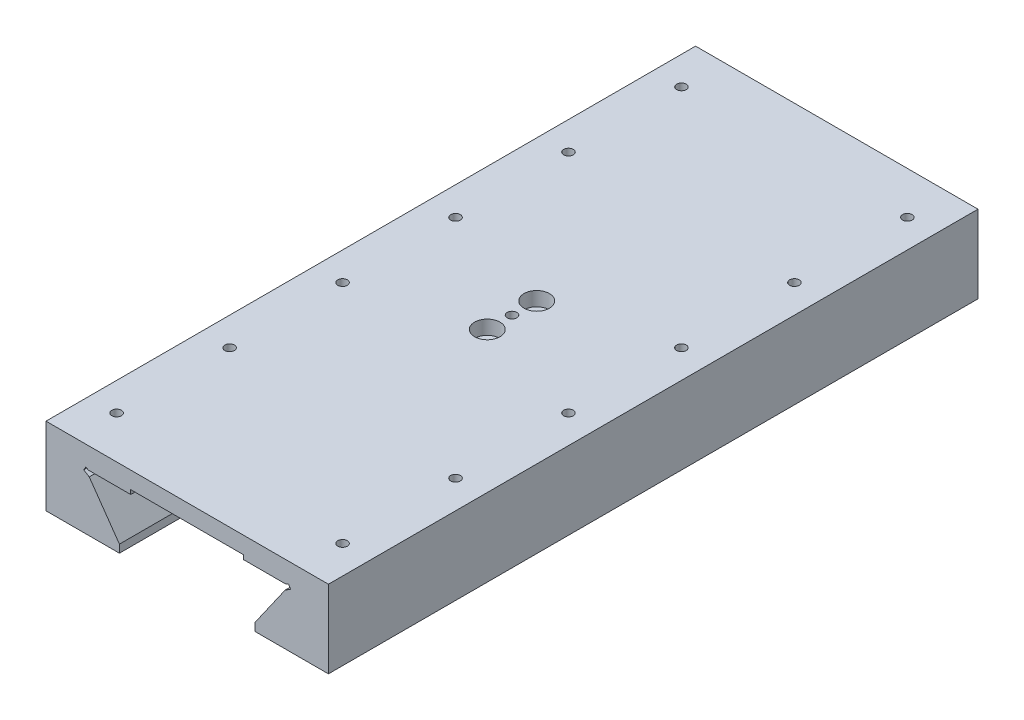
from build123d import *

# Parameters (mm, degrees)
BOSS_EXTRUDE1_DEPTH                     = 460
CBORE_FOR_M8_HEX_HEAD_BOLT1_D           = 9
CBORE_FOR_M8_HEX_HEAD_BOLT1_CBORE_D     = 18
CBORE_FOR_M8_HEX_HEAD_BOLT1_CBORE_DEPTH = 10
M8_TAPPED_HOLE1_D                       = 6.8
M8_TAPPED_HOLE1_DEPTH                   = 19.75
M8_TAPPED_HOLE1_TIP                     = 2.042926105


with BuildPart() as part:
    # Sketch1 → Boss-Extrude1 (new body)
    with BuildSketch(Plane.XY):
        Polygon((-40, 52.5), (-40, 55.5), (40, 55.5), (40, 52.5), (70, 52.5), (71.711448084, 53.534864946), (73.263745503, 50.96769282), (69.385770597, 48.622789502), (48, 18.080743852), (48, 12.5), (100, 12.5), (100, 67.5), (-100, 67.5), (-100, 12.5), (-48, 12.5), (-48, 18.080743852), (-69.385770597, 48.622789502), (-73.263745503, 50.96769282), (-71.711448084, 53.534864946), (-70, 52.5), align=None)
    extrude(amount=-BOSS_EXTRUDE1_DEPTH)

    # CBORE for M8 Hex Head Bolt1 (through all)
    with Locations(Plane(origin=(0, 67.5, 0), x_dir=(1, 0, 0), z_dir=(0, 1, 0))):
        with Locations((0, 247.5), (0, 212.5)):
            CounterBoreHole(CBORE_FOR_M8_HEX_HEAD_BOLT1_D / 2, CBORE_FOR_M8_HEX_HEAD_BOLT1_CBORE_D / 2, CBORE_FOR_M8_HEX_HEAD_BOLT1_CBORE_DEPTH)

    # M8 Tapped Hole1
    with Locations(Plane(origin=(0, 67.5, 0), x_dir=(1, 0, 0), z_dir=(0, 1, 0))):
        with Locations((1.4e-07, 230), (80.000000279, 430), (-80, 30), (-80, 430), (80.000000279, 30), (-80, 350), (80.000000279, 350), (-80, 270), (80.000000279, 270), (-80, 190), (80.000000279, 190), (-80, 110), (80.000000279, 110)):
            Hole(M8_TAPPED_HOLE1_D / 2, depth=M8_TAPPED_HOLE1_DEPTH)
            with Locations((0, 0, -(M8_TAPPED_HOLE1_DEPTH + M8_TAPPED_HOLE1_TIP / 2))):  # 118° drill point
                Cone(0, M8_TAPPED_HOLE1_D / 2, M8_TAPPED_HOLE1_TIP, mode=Mode.SUBTRACT)


solid = part.part
